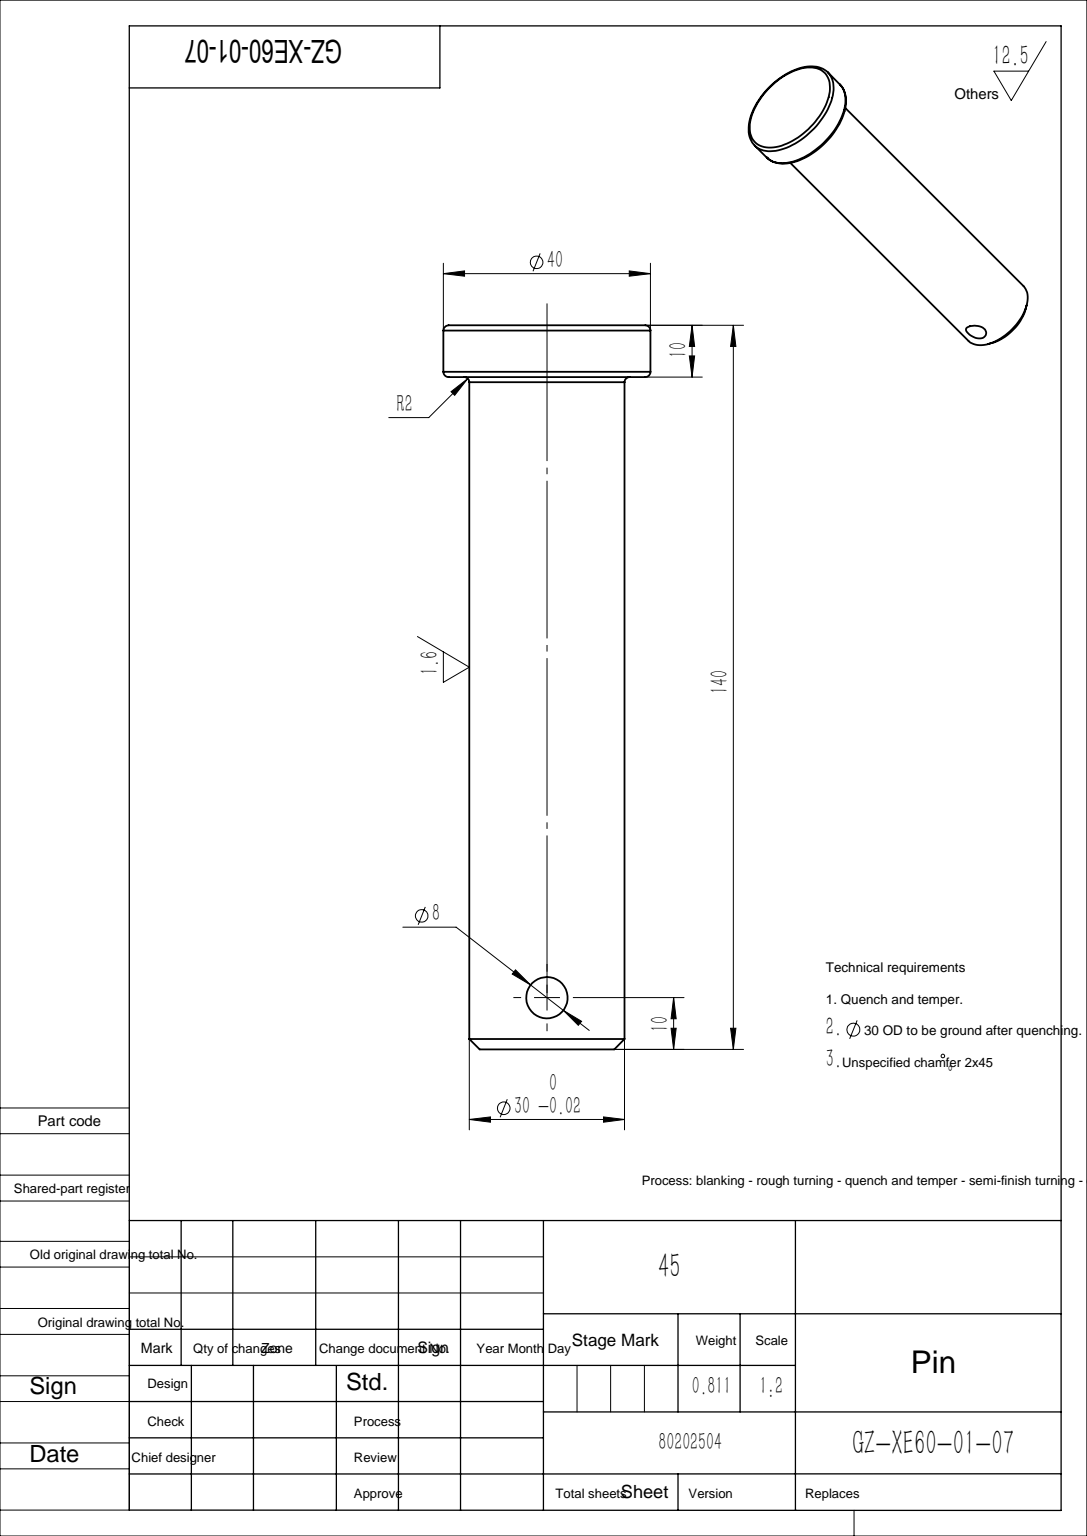
SolidWorks part; units mm, degrees
material "45"
ref_plane "Front Plane" through (0, 0, 0) normal (0, 0, 1) x (1, 0, 0)
ref_plane "Top Plane" through (0, 0, 0) normal (0, 1, 0) x (1, 0, 0)
ref_plane "Right Plane" through (0, 0, 0) normal (1, 0, 0) x (0, 0, -1)
sketch "Sketch1" plane through (0, 0, 0) normal (0, 0, 1) x (1, 0, 0)
  circle A0 centre (0, 0) radius 15
  dimension "D1" = 30
extrude "Boss-Extrude1" add sketch "Sketch1" along normal blind 130
sketch "Sketch2" plane through (0, 0, 130) normal (0, 0, 1) x (1, 0, 0)
  circle A0 centre (0, 0) radius 20
  dimension "D1" = 40
extrude "Boss-Extrude2" add sketch "Sketch2" along normal blind 10
sketch "Sketch3" plane through (0, 0, 0) normal (0, 1, 0) x (1, 0, 0)
  line L0 (15, 0) -> (-15, 0) construction
  circle A0 centre (0, -10) radius 4
  dimension "D1" = 8
  dimension "D2" = 10
extrude "Cut-Extrude1" cut sketch "Sketch3" against normal through all both and the other way through all
chamfer "Chamfer1" distance 2 angle 45 1 edges at (15, 0, 0)
fillet "Fillet1" radius 1 1 edges at (15, 0, 130)
fillet "Fillet2" radius 1 2 edges at (20, 0, 130) (20, 0, 140)
